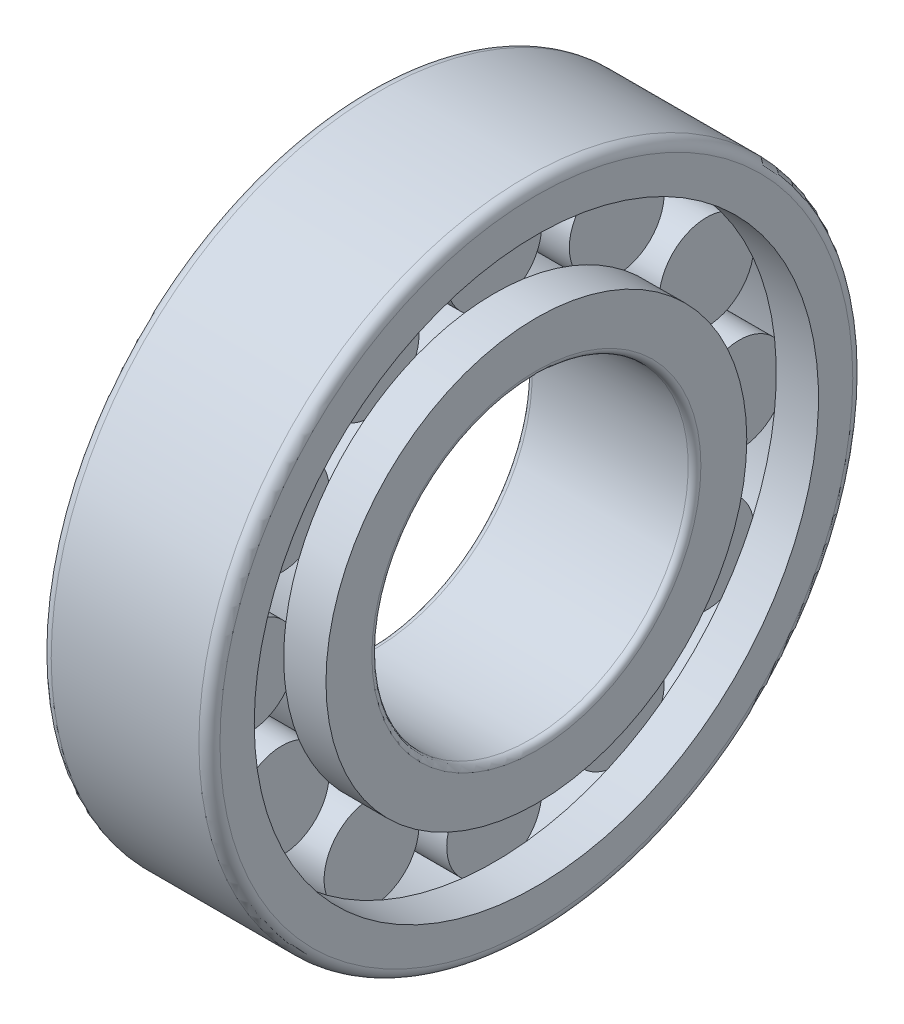
from build123d import *

# Parameters (mm, degrees)
SKETCH_3_W               = 8
SKETCH_3_H               = 4.5001
PATTERN_CIRCULAR_1_COUNT = 12


with BuildPart() as part:
    # 草图2 → Revolve 705 (revolve)
    with BuildSketch(Plane.XY, mode=Mode.PRIVATE) as revolve_705_sk:
        with BuildLine():
            Line((4, 18.75), (12, 18.75))
            Line((12, 18.75), (12, 19.95))
            Line((12, 19.95), (16, 19.95))
            Line((16, 19.95), (16, 15.6))
            ThreePointArc((16, 15.6), (15.824264069, 15.175735931), (15.4, 15))
            Line((15.4, 15), (0.6, 15))
            ThreePointArc((0.6, 15), (0.175735931, 15.175735931), (0, 15.6))
            Line((0, 15.6), (0, 19.95))
            Line((0, 19.95), (4, 19.95))
            Line((4, 19.95), (4, 18.75))
        make_face()
    revolve(revolve_705_sk.sketch.rotate(Axis((-10.080094127, 0, 0), (1, 0, 0)), 90), axis=Axis((-10.080094127, 0, 0), (1, 0, 0)))

    # 草图3 → 凸台-旋转1 (revolve)
    with BuildSketch(Plane.XY):
        with Locations((8, 20.99995)):
            Rectangle(SKETCH_3_W, SKETCH_3_H)
    revolve_1 = revolve(axis=Axis((-1.603948851, 23.25, 0), (1, 0, 0)))

    # 草图4 → 凸台-旋转2 (revolve)
    with BuildSketch(Plane.XY, mode=Mode.PRIVATE) as revolve_2_sk:
        with BuildLine():
            Line((12, 26.75), (16, 26.75))
            Line((16, 26.75), (16, 30))
            ThreePointArc((16, 30), (15.707106781, 30.707106781), (15, 31))
            Line((15, 31), (1, 31))
            ThreePointArc((1, 31), (0.292893219, 30.707106781), (0, 30))
            Line((0, 30), (0, 26.75))
            Line((0, 26.75), (4, 26.75))
            Line((4, 26.75), (4, 27.75))
            Line((4, 27.75), (12, 27.75))
            Line((12, 27.75), (12, 26.75))
        make_face()
    revolve(revolve_2_sk.sketch.rotate(Axis((0, 0, 0), (1, 0, 0)), 90), axis=Axis((0, 0, 0), (1, 0, 0)))

    # 阵列(圆周)1: 凸台-旋转1 ×12 about axis
    pattern_circular_1_axis = Axis((0, 0, 0), (1, 0, 0))
    for i in range(1, PATTERN_CIRCULAR_1_COUNT):
        add(revolve_1.rotate(pattern_circular_1_axis, i * 360 / PATTERN_CIRCULAR_1_COUNT))


solid = part.part
